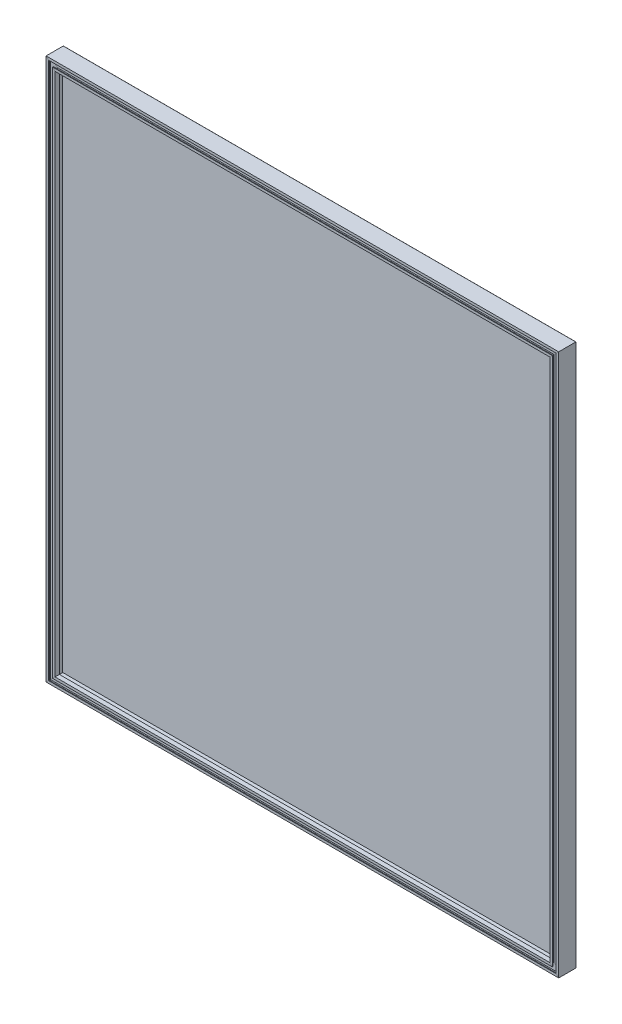
from build123d import *

# Parameters (mm, degrees)
MEMBER_1_DEPTH      = 40.357337308
MEMBER_1_DEPTH_BACK = 1075.357337308
MEMBER_1_2_DEPTH    = 1175.714674617
MEMBER_1_3_DEPTH    = 1115.714674617
MEMBER_1_4_DEPTH    = 1175.714674617
SKETCH_12_W         = 1025
SKETCH_12_H         = 1085
EXTRUDE_1_DEPTH     = 3


with BuildPart() as part:
    # 草图11 → Member 1 (new, two sides: drawn at the far end of the back side and taken through both)
    with BuildSketch(Plane(origin=(-517.5, 547.5, 0), x_dir=(0, -1, 0), z_dir=(-1, 0, 0)).offset(-MEMBER_1_DEPTH_BACK)):
        with BuildLine():
            Line((13, -1.5), (13, 0))
            Line((13, 0), (18, 0))
            Line((18, 0), (18, -8.7))
            Line((18, -8.7), (2, -8.7))
            Line((2, -8.7), (2, -32))
            ThreePointArc((2, -32), (2.292893219, -32.707106781), (3, -33))
            Line((3, -33), (8, -33))
            Line((8, -33), (8, -31.5))
            Line((8, -31.5), (10, -31.5))
            Line((10, -31.5), (10, -35))
            Line((10, -35), (0.5, -35))
            ThreePointArc((0.5, -35), (0.146446609, -34.853553391), (0, -34.5))
            Line((0, -34.5), (0, 0))
            Line((0, 0), (5, 0))
            Line((5, 0), (5, -1.5))
            Line((5, -1.5), (2, -1.5))
            Line((2, -1.5), (2, -6.7))
            Line((2, -6.7), (16, -6.7))
            Line((16, -6.7), (16, -1.5))
            Line((16, -1.5), (13, -1.5))
        make_face()
    extrude(amount=MEMBER_1_DEPTH + MEMBER_1_DEPTH_BACK)

    # Member 1 mitre 1
    split(bisect_by=Plane(origin=(-517.5, 547.5, 0), x_dir=(-0.707106781, 0.707106781, 0), z_dir=(0.707106781, 0.707106781, 0)), keep=Keep.TOP)

    # Member 1 mitre 2
    split(bisect_by=Plane(origin=(517.5, 547.5, 0), x_dir=(-0.707106781, -0.707106781, 0), z_dir=(-0.707106781, 0.707106781, 0)), keep=Keep.TOP)


with BuildPart() as body_2:
    # 草图11 on segment 2 (carried to segment 2) → Member 1 2 (new body)
    with BuildSketch(Plane(origin=(517.5, -587.857337308, 0), x_dir=(-1, 0, 0), z_dir=(0, 1, 0))):
        with BuildLine():
            Line((13, -1.5), (13, 0))
            Line((13, 0), (18, 0))
            Line((18, 0), (18, -8.7))
            Line((18, -8.7), (2, -8.7))
            Line((2, -8.7), (2, -32))
            ThreePointArc((2, -32), (2.292893219, -32.707106781), (3, -33))
            Line((3, -33), (8, -33))
            Line((8, -33), (8, -31.5))
            Line((8, -31.5), (10, -31.5))
            Line((10, -31.5), (10, -35))
            Line((10, -35), (0.5, -35))
            ThreePointArc((0.5, -35), (0.146446609, -34.853553391), (0, -34.5))
            Line((0, -34.5), (0, 0))
            Line((0, 0), (5, 0))
            Line((5, 0), (5, -1.5))
            Line((5, -1.5), (2, -1.5))
            Line((2, -1.5), (2, -6.7))
            Line((2, -6.7), (16, -6.7))
            Line((16, -6.7), (16, -1.5))
            Line((16, -1.5), (13, -1.5))
        make_face()
    extrude(amount=MEMBER_1_2_DEPTH)

    # Member 1 2 mitre 1
    split(bisect_by=Plane(origin=(517.5, 547.5, 0), x_dir=(0.707106781, 0.707106781, 0), z_dir=(0.707106781, -0.707106781, 0)), keep=Keep.TOP)

    # Member 1 2 mitre 2
    split(bisect_by=Plane(origin=(517.5, -547.5, 0), x_dir=(-0.707106781, 0.707106781, 0), z_dir=(0.707106781, 0.707106781, 0)), keep=Keep.TOP)


with BuildPart() as body_3:
    # 草图11 on segment 3 (carried to segment 3) → Member 1 3 (new body)
    with BuildSketch(Plane(origin=(-557.857337308, -547.5, 0), x_dir=(0, 1, 0), z_dir=(1, 0, 0))):
        with BuildLine():
            Line((13, -1.5), (13, 0))
            Line((13, 0), (18, 0))
            Line((18, 0), (18, -8.7))
            Line((18, -8.7), (2, -8.7))
            Line((2, -8.7), (2, -32))
            ThreePointArc((2, -32), (2.292893219, -32.707106781), (3, -33))
            Line((3, -33), (8, -33))
            Line((8, -33), (8, -31.5))
            Line((8, -31.5), (10, -31.5))
            Line((10, -31.5), (10, -35))
            Line((10, -35), (0.5, -35))
            ThreePointArc((0.5, -35), (0.146446609, -34.853553391), (0, -34.5))
            Line((0, -34.5), (0, 0))
            Line((0, 0), (5, 0))
            Line((5, 0), (5, -1.5))
            Line((5, -1.5), (2, -1.5))
            Line((2, -1.5), (2, -6.7))
            Line((2, -6.7), (16, -6.7))
            Line((16, -6.7), (16, -1.5))
            Line((16, -1.5), (13, -1.5))
        make_face()
    extrude(amount=MEMBER_1_3_DEPTH)

    # Member 1 3 mitre 1
    split(bisect_by=Plane(origin=(-517.5, -547.5, 0), x_dir=(0.707106781, 0.707106781, 0), z_dir=(0.707106781, -0.707106781, 0)), keep=Keep.TOP)

    # Member 1 3 mitre 2
    split(bisect_by=Plane(origin=(517.5, -547.5, 0), x_dir=(0.707106781, -0.707106781, 0), z_dir=(-0.707106781, -0.707106781, 0)), keep=Keep.TOP)


with BuildPart() as body_4:
    # 草图11 on segment 4 (carried to segment 4) → Member 1 4 (new body)
    with BuildSketch(Plane(origin=(-517.5, 587.857337308, 0), x_dir=(1, 0, 0), z_dir=(0, -1, 0))):
        with BuildLine():
            Line((13, -1.5), (13, 0))
            Line((13, 0), (18, 0))
            Line((18, 0), (18, -8.7))
            Line((18, -8.7), (2, -8.7))
            Line((2, -8.7), (2, -32))
            ThreePointArc((2, -32), (2.292893219, -32.707106781), (3, -33))
            Line((3, -33), (8, -33))
            Line((8, -33), (8, -31.5))
            Line((8, -31.5), (10, -31.5))
            Line((10, -31.5), (10, -35))
            Line((10, -35), (0.5, -35))
            ThreePointArc((0.5, -35), (0.146446609, -34.853553391), (0, -34.5))
            Line((0, -34.5), (0, 0))
            Line((0, 0), (5, 0))
            Line((5, 0), (5, -1.5))
            Line((5, -1.5), (2, -1.5))
            Line((2, -1.5), (2, -6.7))
            Line((2, -6.7), (16, -6.7))
            Line((16, -6.7), (16, -1.5))
            Line((16, -1.5), (13, -1.5))
        make_face()
    extrude(amount=MEMBER_1_4_DEPTH)

    # Member 1 4 mitre 1
    split(bisect_by=Plane(origin=(-517.5, 547.5, 0), x_dir=(0.707106781, -0.707106781, 0), z_dir=(-0.707106781, -0.707106781, 0)), keep=Keep.TOP)

    # Member 1 4 mitre 2
    split(bisect_by=Plane(origin=(-517.5, -547.5, 0), x_dir=(-0.707106781, -0.707106781, 0), z_dir=(-0.707106781, 0.707106781, 0)), keep=Keep.TOP)


with BuildPart() as body_5:
    # 草图12 → 凸台-拉伸1 (new body)
    with BuildSketch(Plane.XY.offset(-31.5)):
        Rectangle(SKETCH_12_W, SKETCH_12_H)
    extrude(amount=EXTRUDE_1_DEPTH)


solid = Compound([part.part, body_2.part, body_3.part, body_4.part, body_5.part])
